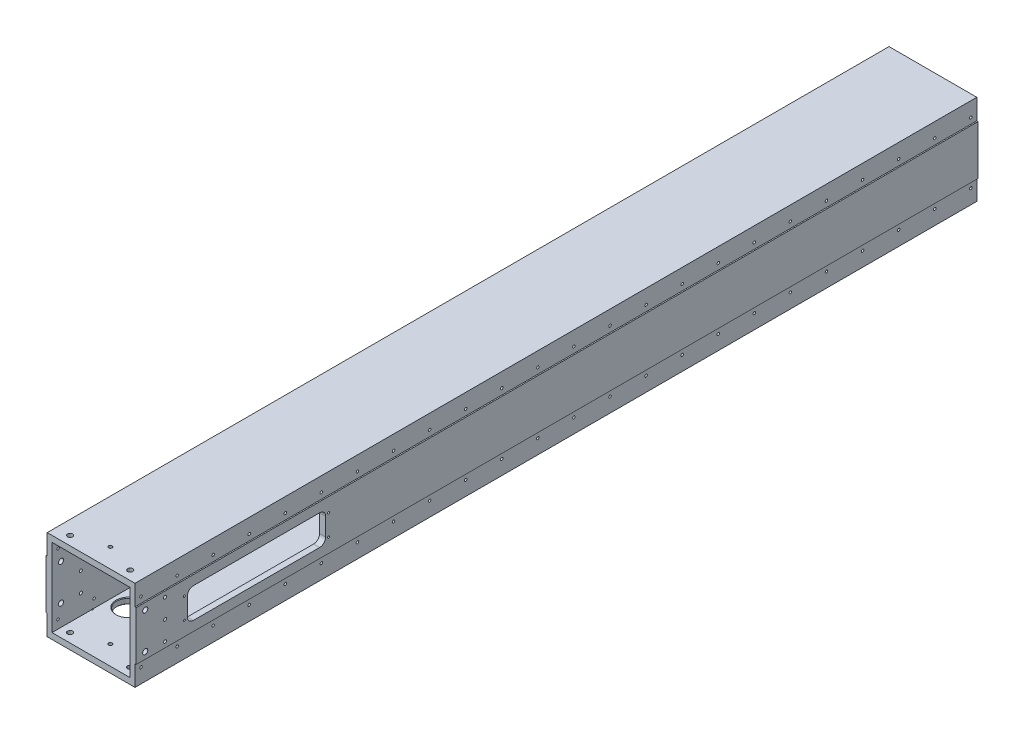
from build123d import *

# Parameters (mm, degrees)
SKETCH_1_W             = 150
SKETCH_1_H             = 150
SKETCH_1_W_2           = 130
SKETCH_1_H_2           = 130
EXTRUDE_1_DEPTH        = 700
SKETCH_2_W             = 2
SKETCH_2_H             = 34
CUT_EXTRUDE_1_DEPTH    = 1405.01210821
HOLE_WIZARD_M8_5_D     = 6.8
HOLE_WIZARD_M8_5_DEPTH = 10
HOLE_WIZARD_M10_2_D    = 8.5
HOLE_WIZARD_M5_3_D     = 4.2
HOLE_WIZARD_M5_4_D     = 4.2
HOLE_WIZARD_M5_4_DEPTH = 12.4
HOLE_WIZARD_M5_4_TIP   = 1.2618073
HOLE_WIZARD_M10_1_D    = 8.5
HOLE_WIZARD_M4_1_D     = 3.3
HOLE_WIZARD_M4_1_DEPTH = 10.1
HOLE_WIZARD_M4_1_TIP   = 0.991420021
CUT_EXTRUDE_2_REACH    = 721.809
SKETCH_23_R            = 20
HOLE_WIZARD_M5_5_D     = 4.2
HOLE_WIZARD_M5_5_DEPTH = 10
HOLE_WIZARD_M6_1_D     = 5
CHAMFER_1_SIZE         = 1
CUT_EXTRUDE_3_REACH    = 721.809
SKETCH_28_W            = 230
SKETCH_28_H            = 50
FILLET_1_R             = 10
HOLE_WIZARD_M4_2_D     = 3.3
HOLE_WIZARD_M4_3_D     = 3.3
HOLE_WIZARD_M4_3_DEPTH = 10
HOLE_WIZARD_M8_7_D     = 6.8
HOLE_WIZARD_M8_7_DEPTH = 10
F_6_0MM_1_D            = 6


with BuildPart() as part:
    # 草图1 → 凸台-拉伸1 (new, symmetric)
    with BuildSketch(Plane.XY):
        Rectangle(SKETCH_1_W, SKETCH_1_H)
        Rectangle(SKETCH_1_W_2, SKETCH_1_H_2, mode=Mode.SUBTRACT)
    extrude(amount=EXTRUDE_1_DEPTH, both=True)

    # 草图2 → 切除-拉伸1 (cut, through all)
    with BuildSketch(Plane.XY.offset(700)):
        with Locations((-74, 58)):
            Rectangle(SKETCH_2_W, SKETCH_2_H)
        with Locations((74, 58)):
            Rectangle(SKETCH_2_W, SKETCH_2_H)
        with Locations((74, -58)):
            Rectangle(SKETCH_2_W, SKETCH_2_H)
        with Locations((-74, -58)):
            Rectangle(SKETCH_2_W, SKETCH_2_H)
    extrude(amount=-CUT_EXTRUDE_1_DEPTH, mode=Mode.SUBTRACT)

    # M8 螺纹孔5
    with Locations(Plane(origin=(0, -75, 0), x_dir=(-1, 0, 0), z_dir=(0, -1, 0))):
        with Locations((-37.5, -552), (37.5, -552)):
            Hole(HOLE_WIZARD_M8_5_D / 2, depth=HOLE_WIZARD_M8_5_DEPTH)

    # M10 螺纹孔2 (through all)
    with Locations(Plane(origin=(75, 0, 0), x_dir=(0, 0, -1), z_dir=(1, 0, 0))):
        with Locations((-685, 30), (-685, -30)):
            Hole(HOLE_WIZARD_M10_2_D / 2)

    # M5 螺纹孔3 (through all)
    with Locations(Plane.ZY.offset(73)):
        with Locations((690, 51), (690, -51), (630, 51), (630, -51), (570, 51), (570, -51), (510, 51), (510, -51), (450, 51), (450, -51), (390, 51), (390, -51), (330, 51), (330, -51), (270, 51), (270, -51), (210, 51), (210, -51), (150, 51), (150, -51), (90, 51), (90, -51), (30, 51), (30, -51), (-30, 51), (-30, -51), (-90, 51), (-90, -51), (-150, 51), (-150, -51), (-210, 51), (-210, -51), (-270, 51), (-270, -51), (-330, 51), (-330, -51), (-390, 51), (-390, -51), (-450, 51), (-450, -51), (-510, 51), (-510, -51), (-570, 51), (-570, -51), (-630, 51), (-630, -51), (-690, 51), (-690, -51)):
            Hole(HOLE_WIZARD_M5_3_D / 2)

    # M5 螺纹孔4
    with Locations(Plane(origin=(0, 0, -700), x_dir=(-1, 0, 0), z_dir=(0, 0, -1))):
        with Locations((70, 0), (0, 0), (0, 70), (0, -70), (-70, 0), (-70, 70), (70, 70), (-70, -70), (70, -70)):
            Hole(HOLE_WIZARD_M5_4_D / 2, depth=HOLE_WIZARD_M5_4_DEPTH)
            with Locations((0, 0, -(HOLE_WIZARD_M5_4_DEPTH + HOLE_WIZARD_M5_4_TIP / 2))):  # 118° drill point
                Cone(0, HOLE_WIZARD_M5_4_D / 2, HOLE_WIZARD_M5_4_TIP, mode=Mode.SUBTRACT)

    # M10 螺纹孔1 (through all)
    with Locations(Plane(origin=(0, 75, 0), x_dir=(1, 0, 0), z_dir=(0, 1, 0))):
        with Locations((-50, -685), (50, -685)):
            Hole(HOLE_WIZARD_M10_1_D / 2)

    # M4 螺纹孔1
    with Locations(Plane(origin=(0, -75, 0), x_dir=(-1, 0, 0), z_dir=(0, -1, 0))):
        with Locations((65.5, -493), (65.5, -293), (65.5, -93), (65.5, 107), (65.5, 307), (65.5, 507), (65.5, 707), (-65.5, 707), (-65.5, 507), (-65.5, 307), (-65.5, 107), (-65.5, -93), (-65.5, -293), (-65.5, -493), (65.5, -563), (-65.5, -563), (65.5, -633), (-65.5, -633)):
            Hole(HOLE_WIZARD_M4_1_D / 2, depth=HOLE_WIZARD_M4_1_DEPTH)
            with Locations((0, 0, -(HOLE_WIZARD_M4_1_DEPTH + HOLE_WIZARD_M4_1_TIP / 2))):  # 118° drill point
                Cone(0, HOLE_WIZARD_M4_1_D / 2, HOLE_WIZARD_M4_1_TIP, mode=Mode.SUBTRACT)

    # 草图23 → 切除-拉伸2 (cut, up to next)
    with BuildSketch(Plane.XZ.offset(75), mode=Mode.PRIVATE) as cut_extrude_2_sk1:
        with Locations(Location((37.5, 600, 0), (0, 0, 270))):
            Circle(SKETCH_23_R)
    cut_extrude_2_tool1 = extrude(cut_extrude_2_sk1.sketch, amount=-CUT_EXTRUDE_2_REACH, mode=Mode.PRIVATE) & part.part
    # 草图23 → 切除-拉伸2 (cut, up to next)
    with BuildSketch(Plane.XZ.offset(75), mode=Mode.PRIVATE) as cut_extrude_2_sk2:
        with Locations(Location((-37.5, 600, 0), (0, 0, 90))):
            Circle(SKETCH_23_R)
    cut_extrude_2_tool2 = extrude(cut_extrude_2_sk2.sketch, amount=-CUT_EXTRUDE_2_REACH, mode=Mode.PRIVATE) & part.part
    add(cut_extrude_2_tool1.solids().sort_by_distance((37.5, -75, 600))[0], mode=Mode.SUBTRACT)
    add(cut_extrude_2_tool2.solids().sort_by_distance((-37.5, -75, 600))[0], mode=Mode.SUBTRACT)

    # M5 螺纹孔5
    with Locations(Plane(origin=(0, -75, 0), x_dir=(-1, 0, 0), z_dir=(0, -1, 0))):
        with Locations((-65, -552), (65, -552)):
            Hole(HOLE_WIZARD_M5_5_D / 2, depth=HOLE_WIZARD_M5_5_DEPTH)

    # M6 螺纹孔1 (through all)
    with Locations(Plane(origin=(75, 0, 0), x_dir=(0, 0, -1), z_dir=(1, 0, 0))):
        with Locations((-652, 32), (-652, 0), (-652, -32)):
            Hole(HOLE_WIZARD_M6_1_D / 2)

    # 倒角1
    chamfer_1_edges = [part.edges().sort_by_distance(p)[0] for p in [
        (37.5, -65, 620),
        (37.5, -75, 620),
        (-37.5, -65, 580),
        (-37.5, -75, 580),
    ]]
    chamfer(chamfer_1_edges, length=CHAMFER_1_SIZE)

    # 草图28 → 切除-拉伸3 (cut, up to next)
    with BuildSketch(Plane(origin=(75, 0, 0), x_dir=(0, 0, -1), z_dir=(1, 0, 0)), mode=Mode.PRIVATE) as cut_extrude_3_sk1:
        with Locations((-500, 0)):
            Rectangle(SKETCH_28_W, SKETCH_28_H)
    cut_extrude_3_tool1 = extrude(cut_extrude_3_sk1.sketch, amount=-CUT_EXTRUDE_3_REACH, mode=Mode.PRIVATE) & part.part
    add(cut_extrude_3_tool1.solids().sort_by_distance((75, 0, 500))[0], mode=Mode.SUBTRACT)

    # 圆角1
    fillet_1_edges = [part.edges().sort_by_distance(p)[0] for p in [
        (70, 25, 615),
        (70, -25, 615),
        (70, -25, 385),
        (70, 25, 385),
    ]]
    fillet(fillet_1_edges, radius=FILLET_1_R)

    # M4 螺纹孔2 (through all)
    with Locations(Plane(origin=(73, 0, 0), x_dir=(0, 0, -1), z_dir=(1, 0, 0))):
        with Locations((-595, 0), (-401, 0)):
            Hole(HOLE_WIZARD_M4_2_D / 2)

    # M4 螺纹孔3
    with Locations(Plane(origin=(75, 0, 0), x_dir=(0, 0, -1), z_dir=(1, 0, 0))):
        with Locations((-620, 17.5), (-620, -17.5), (-380, 17.5), (-380, -17.5)):
            Hole(HOLE_WIZARD_M4_3_D / 2, depth=HOLE_WIZARD_M4_3_DEPTH)

    # M8 螺纹孔7
    with Locations(Plane(origin=(0, -75, 0), x_dir=(-1, 0, 0), z_dir=(0, -1, 0))):
        with Locations((-35, -460), (35, -460), (-35, 672), (-35, 653), (35, 672), (35, 653)):
            Hole(HOLE_WIZARD_M8_7_D / 2, depth=HOLE_WIZARD_M8_7_DEPTH)

    # Ø6.0mm 暗销孔1 (through all)
    with Locations(Plane(origin=(0, 75, 0), x_dir=(1, 0, 0), z_dir=(0, 1, 0))):
        with Locations((0, -668)):
            Hole(F_6_0MM_1_D / 2)


solid = part.part
